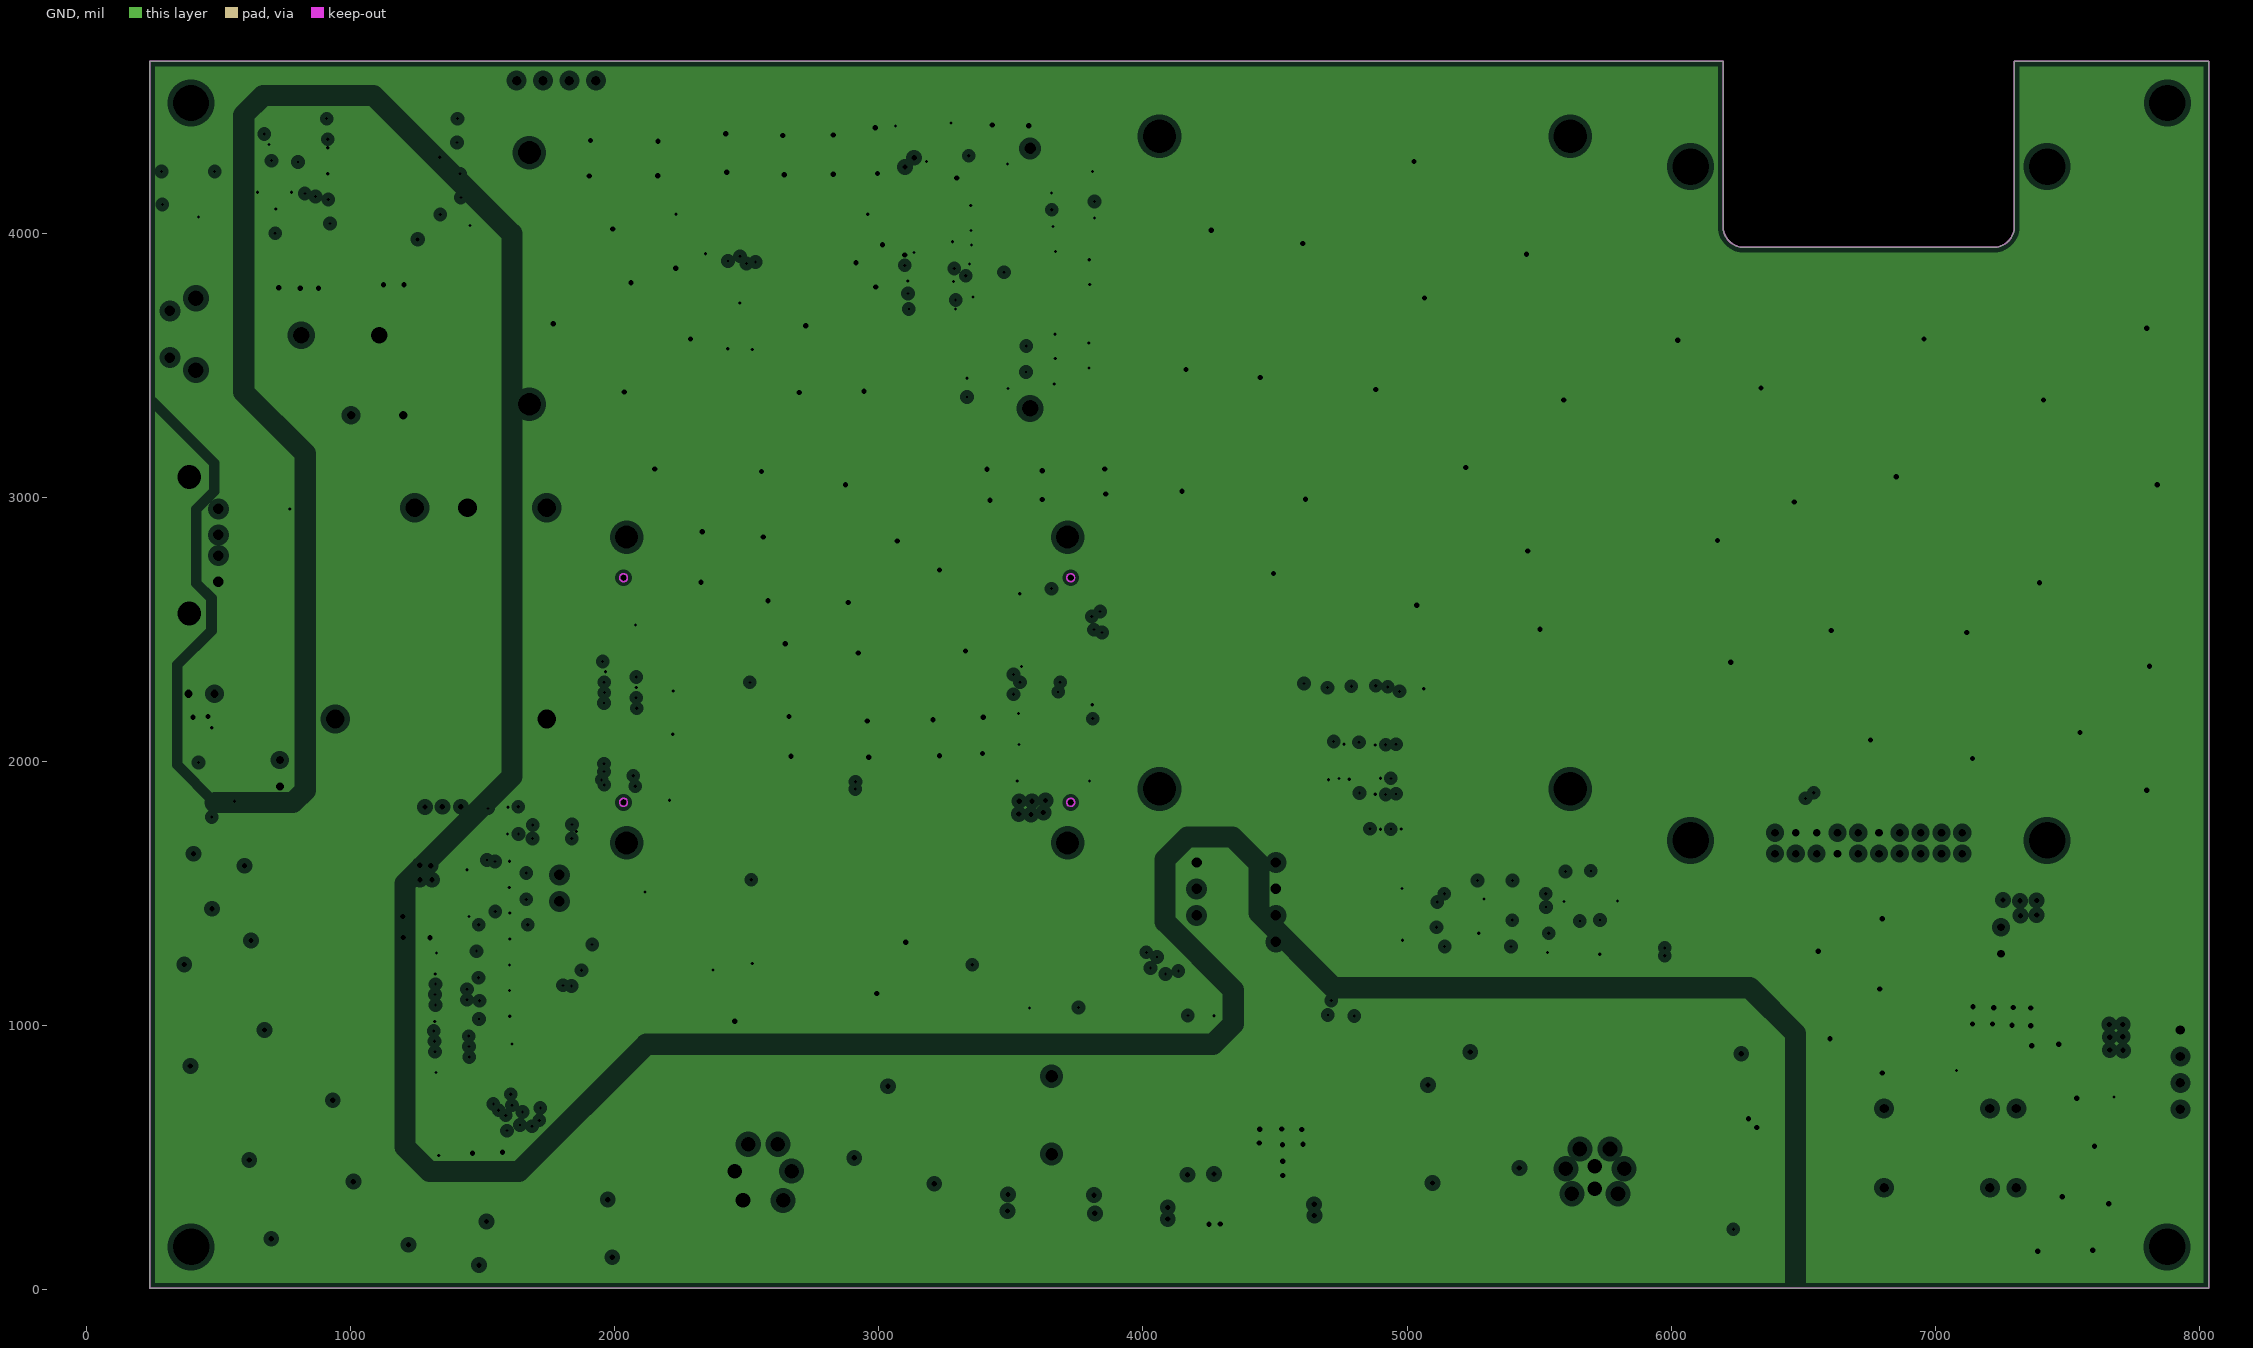
[diagram p0: GND, clearances drawn from the general rule]
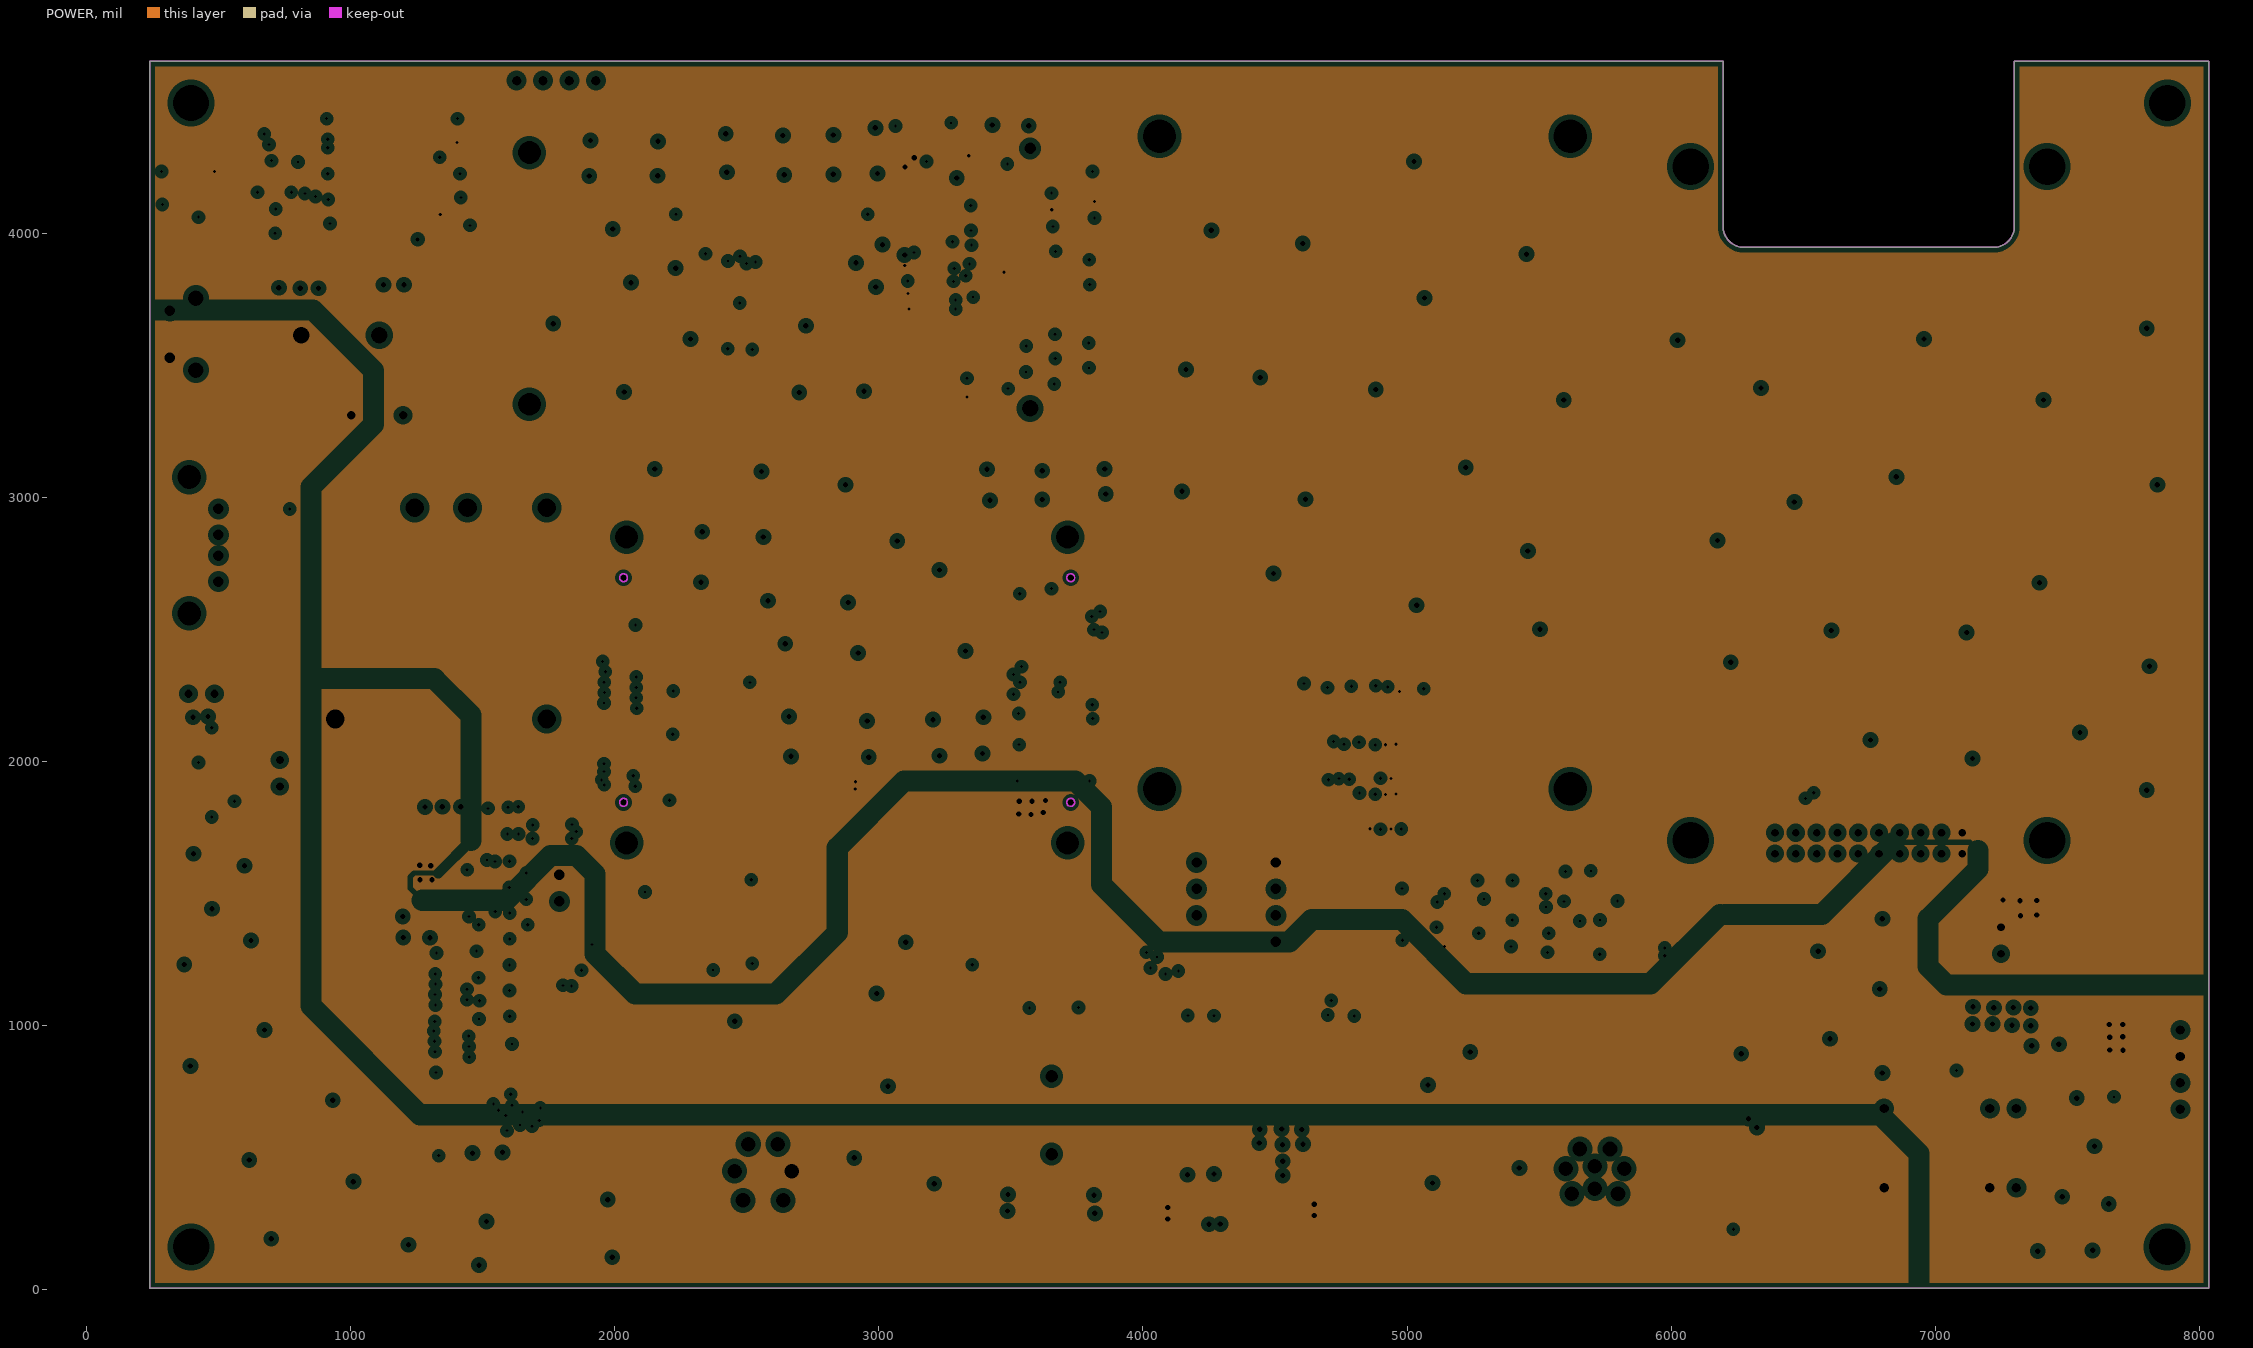
[diagram p1: POWER, clearances drawn from the general rule]
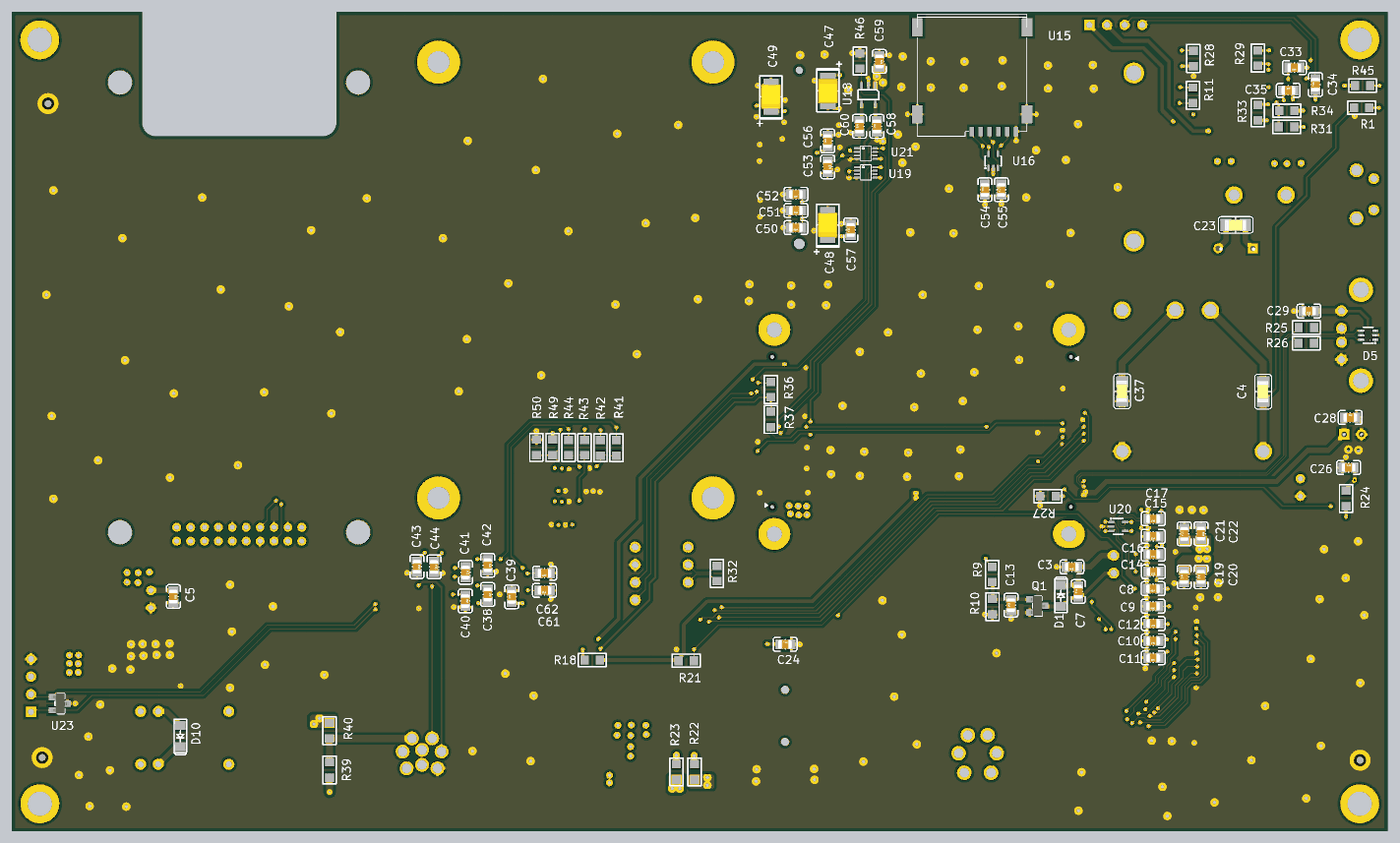
[diagram p2: 3D render of the assembled board from below, using the file's embedded part models]
# Altium PCB MISC82794.PcbDoc (part 2 of 5)
## Footprints (in the part's own frame and the unit in brackets; to place one, negate y for a bottom-side part, rotate by r counter-clockwise, add the part's x,y. Pads: shape width x height; smd on the part's side, far side on the other; paste and mask are expansions set on the pad) (continued)
BATTERY-1220-1 [mm]
  round 1.2 hole 1.2: 0(0,-3.581) 0(0,3.912)
  rect 4x4.5 smd: 1(0,7.62) 2(0,-7.62)
  silkscreen extent -7.22,-7.22 7.22,7.22
BBD-06PMFP-LC7001 [mm]
  round 2.1 hole 1.4: 1(-1.93,2.56) 2(-2.74,-0.25) 3(-1.43,-2.84) 4(1.43,-2.84) 5(2.74,-0.25) 6(1.93,2.56)
  silkscreen extent -11.75,-11.75 11.75,11.75
BDU-08PMFP-LC7001 [mm]
  round 2 hole 1.4: 1(-2.22,1.9) 2(-2.8,-0.5) 3(-1.45,-2.4) 4(1.45,-2.4) 5(2.8,-0.5) 6(2.22,1.9) 7(0,1.4) 8(0,-0.75)
  silkscreen extent -11.75,-11.75 11.75,11.75
C1206 [mm]
  rect 1.6x1.8 smd: 1(-1.4,0) 2(1.4,0)
  silkscreen extent -2.5,-1.2 2.5,1.2, body extent -1.52,-0.82 1.52,0.71, height 0.61
CAPPR5.0-10X16-0.8 [mm]
  rect 1.4x1.4 hole 0.8: 1(-2.5,0)
  round 1.4 hole 0.8: 2(2.5,0)
  silkscreen extent -6.05,-5 5,5, body extent -5.1,-5.1 4.9,4.9, height 15.68
CAPPRD250W45D630H800P [mil] "6.5mm"
  rect 60x60 hole 31.5: 1(-49.21,0)
  round 60 hole 31.5: 2(49.21,0)
  silkscreen extent -124,-124 124,124, body extent -124,-124 124,124, height 453
CT3528-B [mm]
  rect 2x2.2 smd: 1(-1.6,0) 2(1.6,0)
  silkscreen extent -4.2,-1.6 3,1.95, body extent -1.75,-1.4 1.75,1.4, height 1.9
CTM1051AM [mm] "7.7mm"
  round 1.6 hole 1: 1(-3.81,-3.81) 2(-1.27,-3.81) 3(1.27,-3.81) 4(3.81,-3.81) 5(3.81,3.81) 6(1.27,3.81) 7(-1.27,3.81)
  silkscreen extent -6.35,-6.1 6.35,4.81
DO-214 [mm]
  rect 1.8x2.4 smd: 1(-2.3,0) 2(2.3,0)
  silkscreen extent -3.5,-1.9 3.8,1.9
DPAK [mm]
  rect 1.5x2 smd: 1(-2.3,-3.25) 3(2.3,-3.25)
  rect 7x7 smd: 2(0,3.25)
  silkscreen extent -3.68,-1.91 3.68,7.11
E2403UHBDD [mm]
  round 2.5 hole 1.8: 1(-10.16,-2.54) 2(-10.16,2.54) 3(10.16,-10.16) 5(10.16,10.16) 6(-10.16,10.16)
  silkscreen extent -12.7,-12.7 12.7,12.7
FFC0.5-50P-A [mm]
  rect 0.25x2 smd: 1(-12.246,0.645)
  oval 0.25x2 smd: 2(-11.746,0.645) 3(-11.246,0.645) 4(-10.746,0.645) 5(-10.246,0.645) 6(-9.746,0.645) 7(-9.246,0.645) 8(-8.746,0.645) 9(-8.246,0.645) 10(-7.746,0.645) 11(-7.246,0.645) 12(-6.746,0.645) 13(-6.246,0.645) 14(-5.746,0.645) 15(-5.246,0.645) 16(-4.746,0.645) 17(-4.246,0.645) 18(-3.746,0.645) 19(-3.246,0.645) 20(-2.746,0.645) 21(-2.246,0.645) 22(-1.746,0.645) 23(-1.246,0.645) 24(-0.746,0.645) 25(-0.246,0.645) 26(0.254,0.645) 27(0.754,0.645) 28(1.254,0.645) 29(1.754,0.645) 30(2.254,0.645) 31(2.754,0.645) 32(3.254,0.645) 33(3.754,0.645) 34(4.254,0.645) 35(4.754,0.645) 36(5.254,0.645) 37(5.754,0.645) 38(6.254,0.645) 39(6.754,0.645) 40(7.254,0.645) 41(7.754,0.645) 42(8.254,0.645) 43(8.754,0.645) 44(9.254,0.645) 45(9.754,0.645) 46(10.254,0.645) 47(10.754,0.645) 48(11.254,0.645) 49(11.754,0.645) 50(12.254,0.645)
  rect 2.286x3.81 smd: 51(-14.478,-0.645) 52(14.478,-0.645)
  silkscreen extent -15.24,-4.45 15.24,2.52
HDR1X4 [mm] "Connector; Header; 4 Position"
  rect 1.5x1.5 hole 0.9: 1(0,0)
  round 1.5 hole 0.9: 2(2.54,0) 3(5.08,0) 4(7.62,0)
  silkscreen extent -1.27,-1.27 8.89,1.27
HK4100F [mm] "11.8mm"
  round 1.6 hole 0.9: 1(12.7,7.62) 2(0,7.62) 3(0,0) 4(2.54,7.62) 5(2.54,0) 6(12.7,0)
  silkscreen extent -1.27,-1.27 13.97,8.89
HOLE-3.2#1 [mm]
  round 5.6 hole 3.5: 8(0,0)
HOLE-3.2#2 [mm]
  round 5.6 hole 3.5: 8(0.96,3.256)
HOLE-3.2#3 [mm]
  round 5.6 hole 3.5: 8(-5.398,-0.3)
HX-DU1006D [mm]
  round 6.2 hole 3.2: 0(-19.75,0.23) 0(19.75,0.23) 2(-19.75,-62.51) 2(19.75,-62.51)
  rect 0.3x2.1 smd: 1(3.5,-2.35) 2(3.5,2.35) 3(3,-2.35) 4(3,2.35) 5(2.5,-2.35) 6(2.5,2.35) 7(2,-2.35) 8(2,2.35) 9(1.5,-2.35) 10(1.5,2.35) 11(1,-2.35) 12(1,2.35) 13(0.5,-2.35) 14(0.5,2.35) 15(0,-2.35) 16(0,2.35) 17(-0.5,-2.35) 18(-0.5,2.35) 19(-1,-2.35) 20(-1,2.35) 21(-1.5,-2.35) 22(-1.5,2.35) 23(-2,-2.35) 24(-2,2.35) 25(-2.5,-2.35) 26(-2.5,2.35) 27(-3,-2.35) 28(-3,2.35) 29(-3.5,-2.35) 30(-3.5,2.35)
  rect 1.6x2.1 smd: 31(-5.9,0) 31(5.9,0)
  silkscreen extent -23.36,-66.07 23.25,3.78
LED0805 [mm]
  rect 1.2x1.3 smd: 1(-1.118,0) 2(1.118,0)
  silkscreen extent -2,-0.95 2.25,0.95
PCIE_0 [mm]
  round 1.6 hole 1.6 unplated: 0(0,0)
  round 3 hole 2.2 unplated: 0(0.4,48.15) 0(24.6,48.15)
  round 1.1 hole 1.1 unplated: 0(25,0)
  rect 0.6x2 smd: 1(0.7,-4.1) 2(1.1,4.1) 3(1.5,-4.1) 4(1.9,4.1) 5(2.3,-4.1) 6(2.7,4.1) 7(3.1,-4.1) 8(3.5,4.1) 9(3.9,-4.1) 10(4.3,4.1) 11(4.7,-4.1) 12(5.1,4.1) 13(5.5,-4.1) 14(5.9,4.1) 15(6.3,-4.1) 16(6.7,4.1) 17(10.3,-4.1) 18(10.7,4.1) 19(11.1,-4.1) 20(11.5,4.1) 21(11.9,-4.1) 22(12.3,4.1) 23(12.7,-4.1) 24(13.1,4.1) 25(13.5,-4.1) 26(13.9,4.1) 27(14.3,-4.1) 28(14.7,4.1) 29(15.1,-4.1) 30(15.5,4.1) 31(15.9,-4.1) 32(16.3,4.1) 33(16.7,-4.1) 34(17.1,4.1) 35(17.5,-4.1) 36(17.9,4.1) 37(18.3,-4.1) 38(18.7,4.1) 39(19.1,-4.1) 40(19.5,4.1) 41(19.9,-4.1) 42(20.3,4.1) 43(20.7,-4.1) 44(21.1,4.1) 45(21.5,-4.1) 46(21.9,4.1) 47(22.3,-4.1) 48(22.7,4.1) 49(23.1,-4.1) 50(23.5,4.1) 51(23.9,-4.1) 52(24.3,4.1)
  rect 2.3x3.2 smd: 53(-2.15,-3.5) 54(27.15,-3.5)
  silkscreen extent -3.43,-6.28 28.45,51.05
RB6.3*7 [mm]
  round 1.35 hole 0.75: 1(-1.27,0) 2(1.27,0)
  silkscreen extent -3.3,-3.3 3.33,3.3
SIM [mm]
  rect 0.65x1.35 smd: 1(-5.07,7.512) 2(-2.53,7.512) 3(0.01,7.512) 5(-6.34,7.512) 6(-3.8,7.512) 7(-1.26,7.512)
  rect 1.55x2.6 smd: 8(-7.9,5.008) 9(7.9,5.008) 10(-7.9,-7.512) 11(7.9,-7.512)
  silkscreen extent -7.9,-9.34 7.9,8.18
SLF6045 [mm]
  rect 1.5x2.2 smd: 1(0.2,3) 2(5.8,3)
  silkscreen extent 0,0 6,6
SMD-4 [mm]
  rect 2x1.5 smd: 1(-4.65,1.27) 2(-4.65,-1.27) 3(4.65,-1.27) 4(4.65,1.27)
  silkscreen extent -5.4,-2.2 3,3, body extent -5.02,-2.42 5.01,2.42, height 3.9
SMD-D4148 [mil]
  rect 50x59.05 smd: 1(-60,0) 2(60,0)
  silkscreen extent -95,-35 106,35
SOIC127P600X175-8N [mil]
  oval 76.06x24 smd: 1(-108.03,75) 2(-108.03,25) 3(-108.03,-25) 4(-108.03,-75) 5(108.03,-75) 6(108.03,-25) 7(108.03,25) 8(108.03,75)
  silkscreen extent -118,-100 50,124, body extent -118,-96 118,97, height 61
SOP16-6.6 [mil]
  rect 80x24 smd: 1(-130,175) 2(-130,125) 3(-130,75) 4(-130,25) 5(-130,-25) 6(-130,-75) 7(-130,-125) 8(-130,-175) 9(130,-175) 10(130,-125) 11(130,-75) 12(130,-25) 13(130,25) 14(130,75) 15(130,125) 16(130,175)
  silkscreen extent -77,-205 77,205
SOT23-5 [mm]
  rect 0.4x1 smd: 1(-1,-1.35) 2(0,-1.35) 3(1,-1.35) 4(1,1.35) 5(-1,1.35)
  silkscreen extent -1.5,-0.7 1.5,0.7
SOT-23 [mil]
  rect 40x36 smd: 1(-42.5,37.4) 2(-42.5,-37.4) 3(42.5,0)
  silkscreen extent -25,-56 25,56, body extent -47,-57 50,58, height 39
SOT-89 [mil]
  rect 39x59 smd: 1(-59,-78.3) 2(0,-78.3) 3(59,-78.3)
  rect 79x79 smd: 2(0,78.3)
  silkscreen extent -100,-79 95,71
SOT-353 [mm]
  rect 0.896x0.35 smd: 1(-1.002,0.65) 2(-1.002,0) 3(-1.002,-0.65) 4(1.002,-0.65) 5(1.002,0.65)
  silkscreen extent -1.14,-1.15 0.7,1.24
SOT-363 [mm]
  rect 0.896x0.35 smd: 1(-1.002,0.65) 2(-1.002,0) 3(-1.002,-0.65) 4(1.002,-0.65) 5(1.002,0) 6(1.002,0.65)
  silkscreen extent -1.14,-1.15 0.7,1.24, body extent -1.15,-1.04 1.15,1.06, height 1
SWICH4.5 [mm] "6.6mm"
  round 1.575 hole 1: 1(2.25,1.25) 2(-2.25,1.25)
  round 2 hole 1.5: 3(-3.45,-1.25) 4(3.45,-1.25)
  silkscreen extent -3.45,-2.75 3.45,6.4
TSOP65P640X120-20N [mm] "TSOP, 20-Leads, Body 6.5x4.4mm (max), Pitch 0.65"
  oval 1.7x0.35 smd: 1(-2.85,2.925) 2(-2.85,2.275) 3(-2.85,1.625) 4(-2.85,0.975) 5(-2.85,0.325) 6(-2.85,-0.325) 7(-2.85,-0.975) 8(-2.85,-1.625) 9(-2.85,-2.275) 10(-2.85,-2.925) 11(2.85,-2.925) 12(2.85,-2.275) 13(2.85,-1.625) 14(2.85,-0.975) 15(2.85,-0.325) 16(2.85,0.325) 17(2.85,0.975) 18(2.85,1.625) 19(2.85,2.275) 20(2.85,2.925)
  silkscreen extent -2.97,-3.25 1.6,3.77, body extent -2.2,-3.25 2.2,3.25, height 1.2
USB-1400 [mm] "5.5mm"
  round 1.6 hole 1: 1(-1.4,-3.5) 2(-1.4,-1) 3(-1.4,1) 4(-1.4,3.5)
  round 3.5 hole 2.3: 5(1.4,6.55) 6(1.4,-6.55)
  silkscreen extent -2.9,-6.9 11.6,6.9
VSSOP-8 [mm]
  rect 0.8x0.3 smd: 1(-1.3,0.75) 2(-1.3,0.25) 3(-1.3,-0.25) 4(-1.3,-0.75) 5(1.3,-0.75) 6(1.3,-0.25) 7(1.3,0.25) 8(1.3,0.75)
  silkscreen extent -0.76,-1.1 0.76,1.1
XH2.5-2P [mm]
  round 1.6 hole 1: 1(2.54,2.54) 2(5.08,2.54)
  silkscreen extent 0.1,-0.01 7.6,5.79